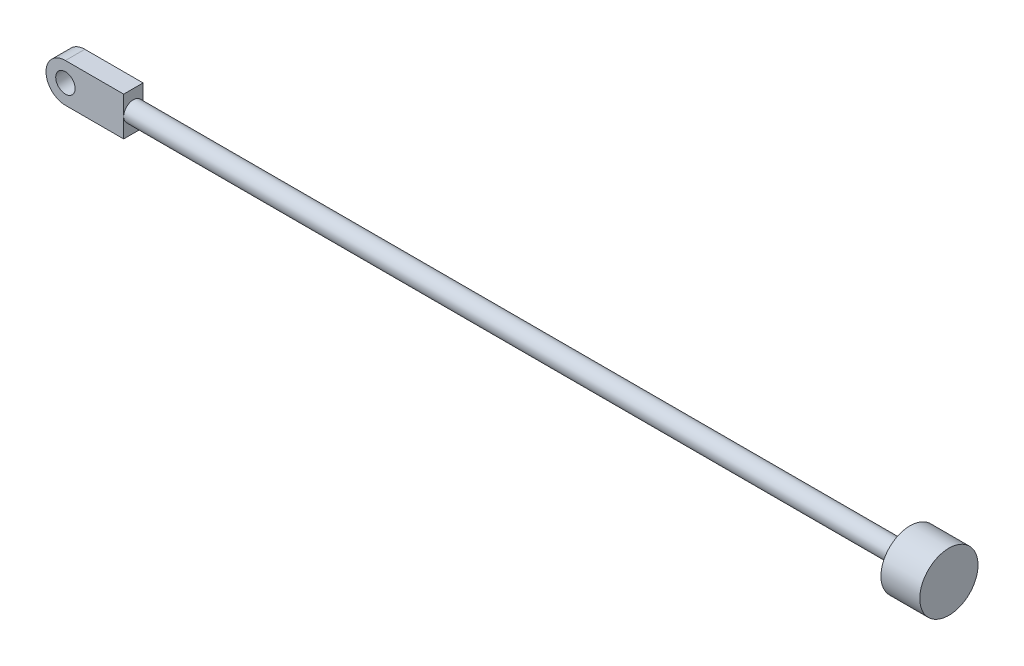
from build123d import *

# Parameters (mm, degrees)
SKETCH1_R           = 5
BOSS_EXTRUDE1_DEPTH = 5


with BuildPart() as part:
    # Sketch1 → Boss-Extrude1 (new, symmetric)
    with BuildSketch(Plane.XY):
        with BuildLine():
            Line((0, 10), (30, 10))
            Line((30, 10), (30, -10))
            Line((30, -10), (0, -10))
            ThreePointArc((0, -10), (-10, 0), (0, 10))
        make_face()
        Circle(SKETCH1_R, mode=Mode.SUBTRACT)
    extrude(amount=BOSS_EXTRUDE1_DEPTH, both=True)

    # Sketch2 → Revolve1 (revolve)
    with BuildSketch(Plane.XY, mode=Mode.PRIVATE) as revolve1_sk:
        Polygon((30, 0), (30, -5), (430, -5), (430, -15), (450, -15), (450, 0), align=None)
    revolve(revolve1_sk.sketch.rotate(Axis((450, 0, 0), (-1, 0, 0)), 180), axis=Axis((450, 0, 0), (-1, 0, 0)))


solid = part.part
